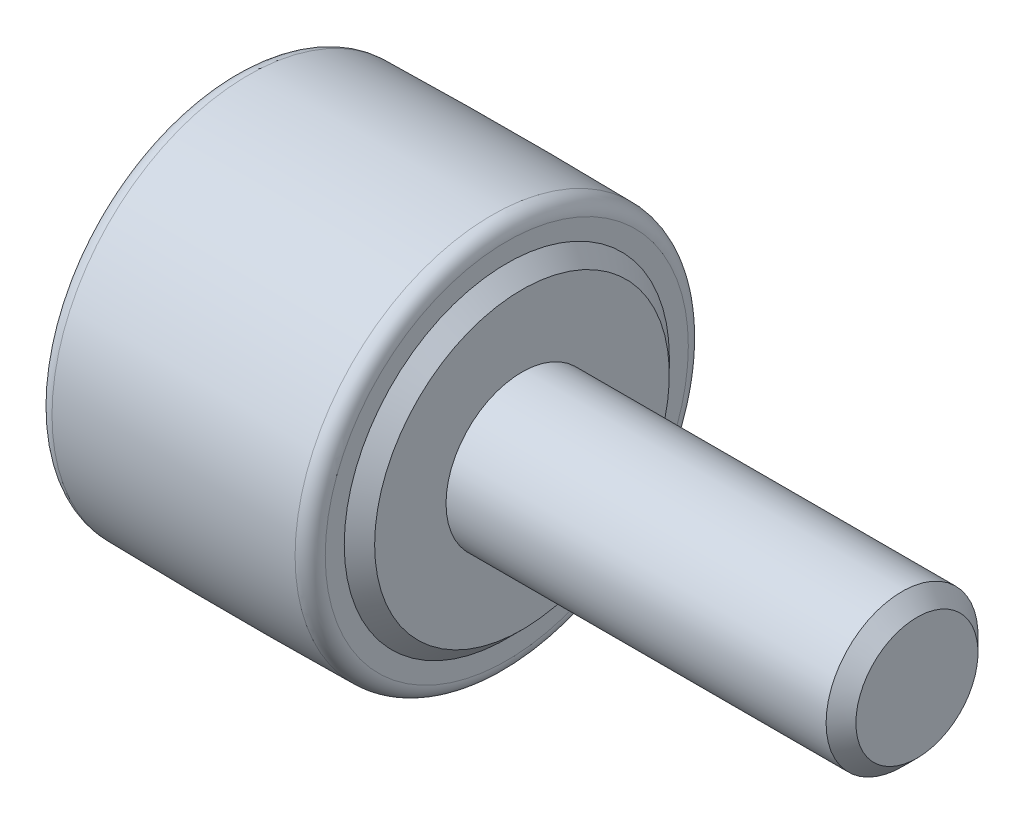
from build123d import *

# Parameters (mm, degrees)
SKETCH2_W          = 6.5
SKETCH2_H          = 1.083333334
CUT_EXTRUDE1_DEPTH = 2


with BuildPart() as part:
    # Sketch1 → Revolve1 (revolve)
    with BuildSketch(Plane.XY, mode=Mode.PRIVATE) as revolve1_sk:
        with BuildLine():
            Line((-10, 0), (-10, 4.85))
            Line((-10, 4.85), (-9.5, 5.35))
            Line((-9.5, 5.35), (-9.5, 5.959415537))
            ThreePointArc((-9.5, 5.959415537), (-9.3567275, 6.309766063), (-9.009018036, 6.459334205))
            ThreePointArc((-9.009018036, 6.459334205), (-5.001066402, 6.499497864), (-0.992985972, 6.475400495))
            ThreePointArc((-0.992985972, 6.475400495), (-0.643975412, 6.326514493), (-0.5, 5.975449694))
            Line((-0.5, 5.975449694), (-0.5, 5.35))
            Line((-0.5, 5.35), (0, 4.85))
            Line((0, 4.85), (0, 2.5))
            Line((0, 2.5), (12.5095, 2.5))
            Line((12.5095, 2.5), (13, 2.0095))
            Line((13, 2.0095), (13, 0))
            Line((13, 0), (-10, 0))
        make_face()
    revolve(revolve1_sk.sketch.rotate(Axis((13, 0, 0), (-1, 0, 0)), 270), axis=Axis((13, 0, 0), (-1, 0, 0)))

    # Sketch2 → Cut-Extrude1 (cut)
    with BuildSketch(Plane.ZY.offset(10)):
        Rectangle(SKETCH2_W, SKETCH2_H)
    extrude(amount=-CUT_EXTRUDE1_DEPTH, mode=Mode.SUBTRACT)


solid = part.part
